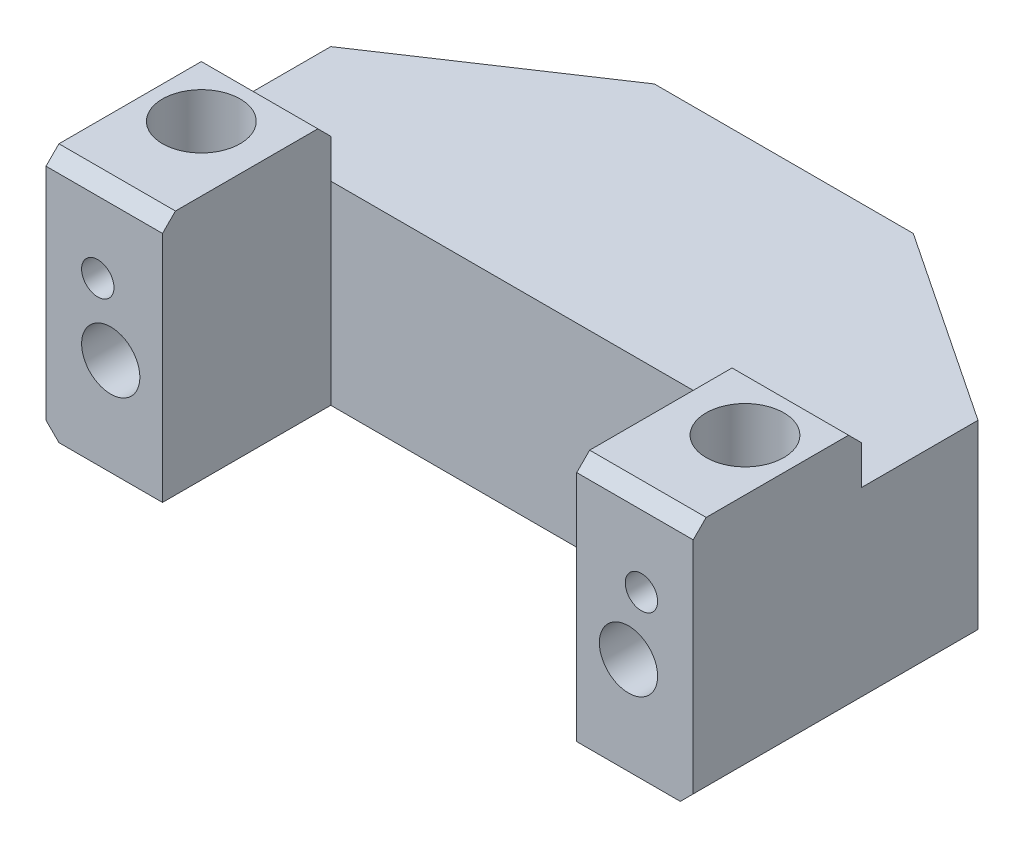
from build123d import *

# Parameters (mm, degrees)
BOSS_EXTRUDE1_DEPTH   = 15
CHAMFER1_SIZE         = 10
CHAMFER1_SIZE2        = 15
CHAMFER2_SIZE         = 15
CHAMFER2_SIZE2        = 10
SKETCH2_R             = 2.25
CUT_EXTRUDE1_DEPTH    = 36
SKETCH3_R             = 4
CUT_EXTRUDE2_DEPTH    = 13
SKETCH12_R            = 3
CUT_EXTRUDE7_DEPTH    = 4.2
M3_TAPPED_HOLE1_D     = 2.5
M3_TAPPED_HOLE1_DEPTH = 7.5
M3_TAPPED_HOLE1_TIP   = 0.751075774
M3_TAPPED_HOLE2_D     = 2.5
M3_TAPPED_HOLE2_DEPTH = 7.5
M3_TAPPED_HOLE2_TIP   = 0.751075774
BOSS_EXTRUDE3_START   = 4
SKETCH17_W            = 9
SKETCH17_H            = 13
SKETCH17_R            = 3
BOSS_EXTRUDE3_DEPTH   = 4
SKETCH18_R            = 5
CUT_EXTRUDE8_DEPTH    = 8.2
CHAMFER3_SIZE         = 1


with BuildPart() as part:
    # Sketch1 → Boss-Extrude1 (new body)
    with BuildSketch(Plane(origin=(0, 0, 0), x_dir=(1, 0, 0), z_dir=(0, 1, 0))):
        Polygon((-25, 16), (25, 16), (25, -16), (16, -16), (16, -3), (-16, -3), (-16, -16), (-25, -16), align=None)
    extrude(amount=BOSS_EXTRUDE1_DEPTH)

    # Chamfer1
    chamfer1_edges = [part.edges().sort_by_distance(p)[0] for p in [
        (25, 7.5, -16),
    ]]
    chamfer1_side = [part.faces().sort_by_distance(p)[0] for p in [
        (25, 7.5, 0),
    ]]
    chamfer(chamfer1_edges, length=CHAMFER1_SIZE, length2=CHAMFER1_SIZE2, reference=chamfer1_side[0])

    # Chamfer2
    chamfer2_edges = [part.edges().sort_by_distance(p)[0] for p in [
        (-25, 7.5, -16),
    ]]
    chamfer2_side = [part.faces().sort_by_distance(p)[0] for p in [
        (-7.5, 7.5, -16),
    ]]
    chamfer(chamfer2_edges, length=CHAMFER2_SIZE, length2=CHAMFER2_SIZE2, reference=chamfer2_side[0])

    # Sketch2 → Cut-Extrude1 (cut)
    with BuildSketch(Plane(origin=(0, 0, -16), x_dir=(-1, 0, 0), z_dir=(0, 0, -1))):
        with Locations((-20, 7.5)):
            Circle(SKETCH2_R)
        with Locations((20, 7.5)):
            Circle(SKETCH2_R)
    extrude(amount=-CUT_EXTRUDE1_DEPTH, mode=Mode.SUBTRACT)

    # Sketch3 → Cut-Extrude2 (cut)
    with BuildSketch(Plane(origin=(0, 0, -16), x_dir=(-1, 0, 0), z_dir=(0, 0, -1))):
        with Locations((-20, 7.5)):
            Circle(SKETCH3_R)
        with Locations((20, 7.5)):
            Circle(SKETCH3_R)
    extrude(amount=-CUT_EXTRUDE2_DEPTH, mode=Mode.SUBTRACT)

    # Sketch12 → Cut-Extrude7 (cut)
    with BuildSketch(Plane(origin=(0, 15, 0), x_dir=(1, 0, 0), z_dir=(0, 1, 0))):
        with Locations(Location((-21, -8, 0), (0, 0, 270))):
            Circle(SKETCH12_R)
        with Locations(Location((21, -8, 0), (0, 0, 270))):
            Circle(SKETCH12_R)
    extrude(amount=-CUT_EXTRUDE7_DEPTH, mode=Mode.SUBTRACT)

    # M3 Tapped Hole1
    with Locations(Plane(origin=(-21, 12.5, 16), x_dir=(1, 0, 0), z_dir=(0, 0, 1))):
        with Locations((0, 0)):
            Hole(M3_TAPPED_HOLE1_D / 2, depth=M3_TAPPED_HOLE1_DEPTH)
            with Locations((0, 0, -(M3_TAPPED_HOLE1_DEPTH + M3_TAPPED_HOLE1_TIP / 2))):  # 118° drill point
                Cone(0, M3_TAPPED_HOLE1_D / 2, M3_TAPPED_HOLE1_TIP, mode=Mode.SUBTRACT)

    # M3 Tapped Hole2
    with Locations(Plane(origin=(21, 12.5, 16), x_dir=(1, 0, 0), z_dir=(0, 0, 1))):
        with Locations((0, 0)):
            Hole(M3_TAPPED_HOLE2_D / 2, depth=M3_TAPPED_HOLE2_DEPTH)
            with Locations((0, 0, -(M3_TAPPED_HOLE2_DEPTH + M3_TAPPED_HOLE2_TIP / 2))):  # 118° drill point
                Cone(0, M3_TAPPED_HOLE2_D / 2, M3_TAPPED_HOLE2_TIP, mode=Mode.SUBTRACT)

    # Sketch17 → Boss-Extrude3 (add)
    # profile 1 of 2: a face of its own
    with BuildSketch(Plane(origin=(0, 15, 0), x_dir=(1, 0, 0), z_dir=(0, 1, 0)).offset(BOSS_EXTRUDE3_START)):
        with Locations((-20.5, -9.5)):
            Rectangle(SKETCH17_W, SKETCH17_H)
        with Locations(Location((-21, -8, 0), (0, 0, 270))):
            Circle(SKETCH17_R, mode=Mode.SUBTRACT)
    # profile 2 of 2: a face of its own
    with BuildSketch(Plane(origin=(0, 15, 0), x_dir=(1, 0, 0), z_dir=(0, 1, 0)).offset(BOSS_EXTRUDE3_START)):
        with Locations((20.5, -9.5)):
            Rectangle(SKETCH17_W, SKETCH17_H)
        with Locations(Location((21, -8, 0), (0, 0, 270))):
            Circle(SKETCH17_R, mode=Mode.SUBTRACT)
    extrude(amount=-BOSS_EXTRUDE3_DEPTH)

    # Sketch18 → Cut-Extrude8 (cut)
    with BuildSketch(Plane.XZ):
        with Locations(Location((0, -7.5, 0), (0, 0, 270))):
            Circle(SKETCH18_R)
    extrude(amount=-CUT_EXTRUDE8_DEPTH, mode=Mode.SUBTRACT)

    # Chamfer3
    chamfer3_edges = [part.edges().sort_by_distance(p)[0] for p in [
        (-20.5, 19, 3),
        (20.5, 19, 3),
        (-20.5, 19, 16),
        (20.5, 19, 16),
        (-25, 0, 5),
        (25, 0, 5),
    ]]
    chamfer(chamfer3_edges, length=CHAMFER3_SIZE)


solid = part.part
